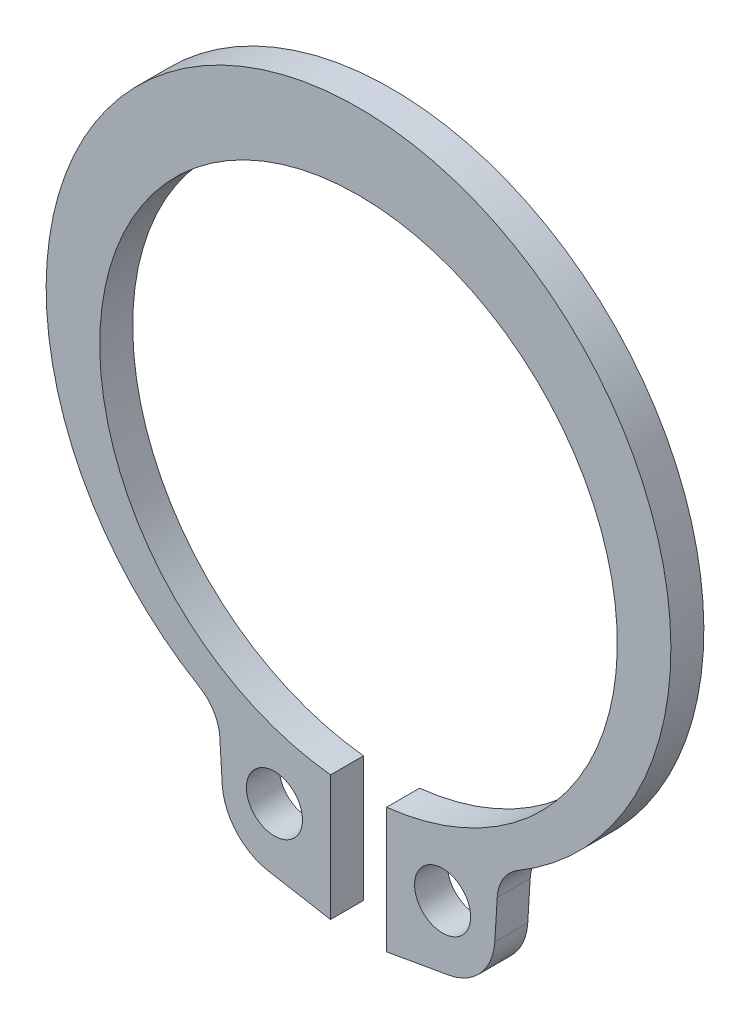
SolidWorks part; units mm, degrees
ref_plane "前视基准面" through (0, 0, 0) normal (0, 0, 1) x (1, 0, 0)
ref_plane "上视基准面" through (0, 0, 0) normal (0, 1, 0) x (1, 0, 0)
ref_plane "右视基准面" through (0, 0, 0) normal (1, 0, 0) x (0, 0, -1)
sketch "草图1" plane through (0, 0, 0) normal (0, 0, 1) x (1, 0, 0)
  line L0 (-12.5, 0) -> (12.5, 0) construction
  line L1 (0, 12.5) -> (0, -12.5) construction
  line L2 (0.85, -7.8038) -> (0.85, -11.6038)
  line L3 (0.85, -11.6038) -> (2.7322, -11.272)
  line L4 (4.1339, -9.7011) -> (4.25, -7.7934)
  circle A0 centre (0, 0) radius 12.5 construction
  circle A1 centre (0, 0) radius 7.85
  circle A2 centre (2.55, -9.4106) radius 0.85
  circle A3 centre (0, 0.675) radius 9.475
  circle A4 centre (0, 0) radius 9.75 construction
  circle A5 centre (0, -0.7435) radius 10.8935 construction
  circle A7 centre (0, 0) radius 8.1 construction
  circle A8 centre (0, 0) radius 8.5 construction
  arc A9 (4.1339, -9.7011) -> (2.7322, -11.272) centre (2.437, -9.5978) cw
  point P8 (0, 10.15)
  point P9 (0, 7.85)
  point P25 (0, -7.85)
  point P26 (0, -8.8)
  dimension "D1" = 1.7
  dimension "d4" = 25
  dimension "d3" = 15.7
  dimension "d5" = 1.7
  dimension "D6" = 1.7
  dimension "D8" = 0.95
  dimension "d2" = 16.2
  dimension "(d1)" = 17
  dimension "D9" = 19.5
  dimension "b" = 2.3
  dimension "a" = 3.8
  dimension "D43" = 5.1
  dimension "D10" = 80
  dimension "D11" = 3.4
sketch "草图2" plane through (0, 0, 0) normal (0, 0, 1) x (1, 0, 0)
  line L0 (4.1339, -9.7011) -> (4.25, -7.7934) construction
  line L1 (0.85, -11.6038) -> (2.7322, -11.272) construction
  line L2 (0.85, -7.8038) -> (0.85, -11.6038) construction
  line L3 (0, 12.5) -> (0, -12.5) construction
  line L4 (4.1339, -9.7011) -> (4.25, -7.7934)
  line L5 (0.85, -11.6038) -> (2.7322, -11.272)
  line L6 (0.85, -7.8038) -> (0.85, -11.6038)
  line L7 (0, 12.5) -> (0, -12.5) construction
  line L8 (-0.85, -11.6038) -> (-2.7322, -11.272)
  line L9 (-4.1339, -9.7011) -> (-4.25, -7.7934)
  line L10 (-0.85, -7.8038) -> (-0.85, -11.6038)
  circle A0 centre (0, 0) radius 7.85 construction
  circle A1 centre (0, 0.675) radius 9.475 construction
  arc A3 (0.85, -7.8038) -> (-0.85, -7.8038) centre (0, 0) ccw
  arc A4 (4.25, -7.7934) -> (-4.25, -7.7934) centre (0, 0.675) ccw
  arc A5 (2.7322, -11.272) -> (4.1339, -9.7011) centre (2.437, -9.5978) ccw construction
  circle A6 centre (2.55, -9.4106) radius 0.85 construction
  circle A7 centre (2.55, -9.4106) radius 0.85
  circle A8 centre (-2.55, -9.4106) radius 0.85
  arc A9 (-2.7322, -11.272) -> (-4.1339, -9.7011) centre (-2.437, -9.5978) cw
  arc A10 (2.7322, -11.272) -> (4.1339, -9.7011) centre (2.437, -9.5978) ccw
extrude "凸台-拉伸1" add sketch "草图2" along normal mid plane 1
fillet "圆角1" radius 1.2667 2 edges at (4.25, -7.7934, 0) (-4.25, -7.7934, 0)
